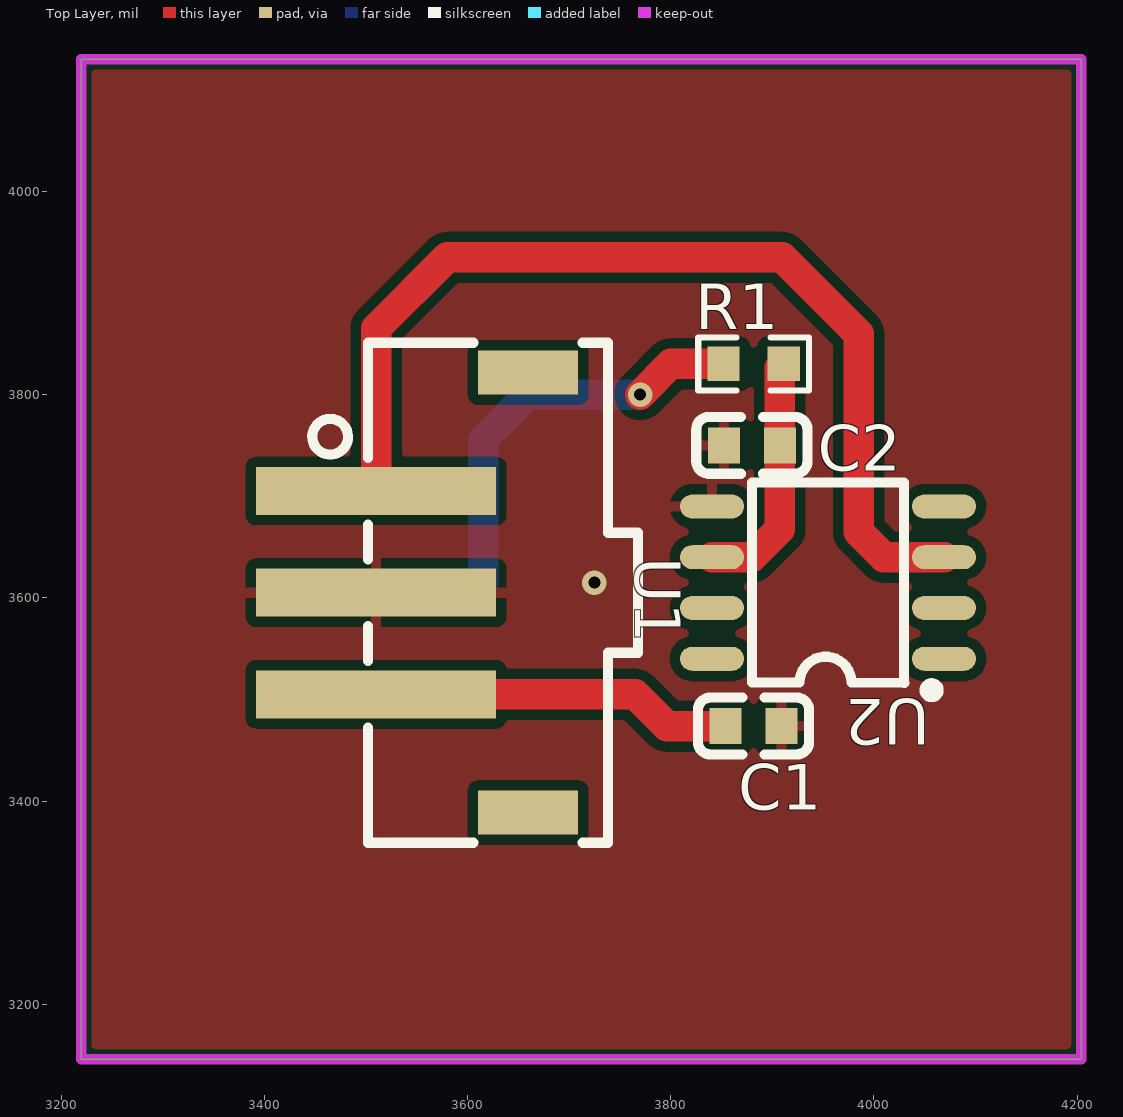
[diagram p0: Top Layer view]
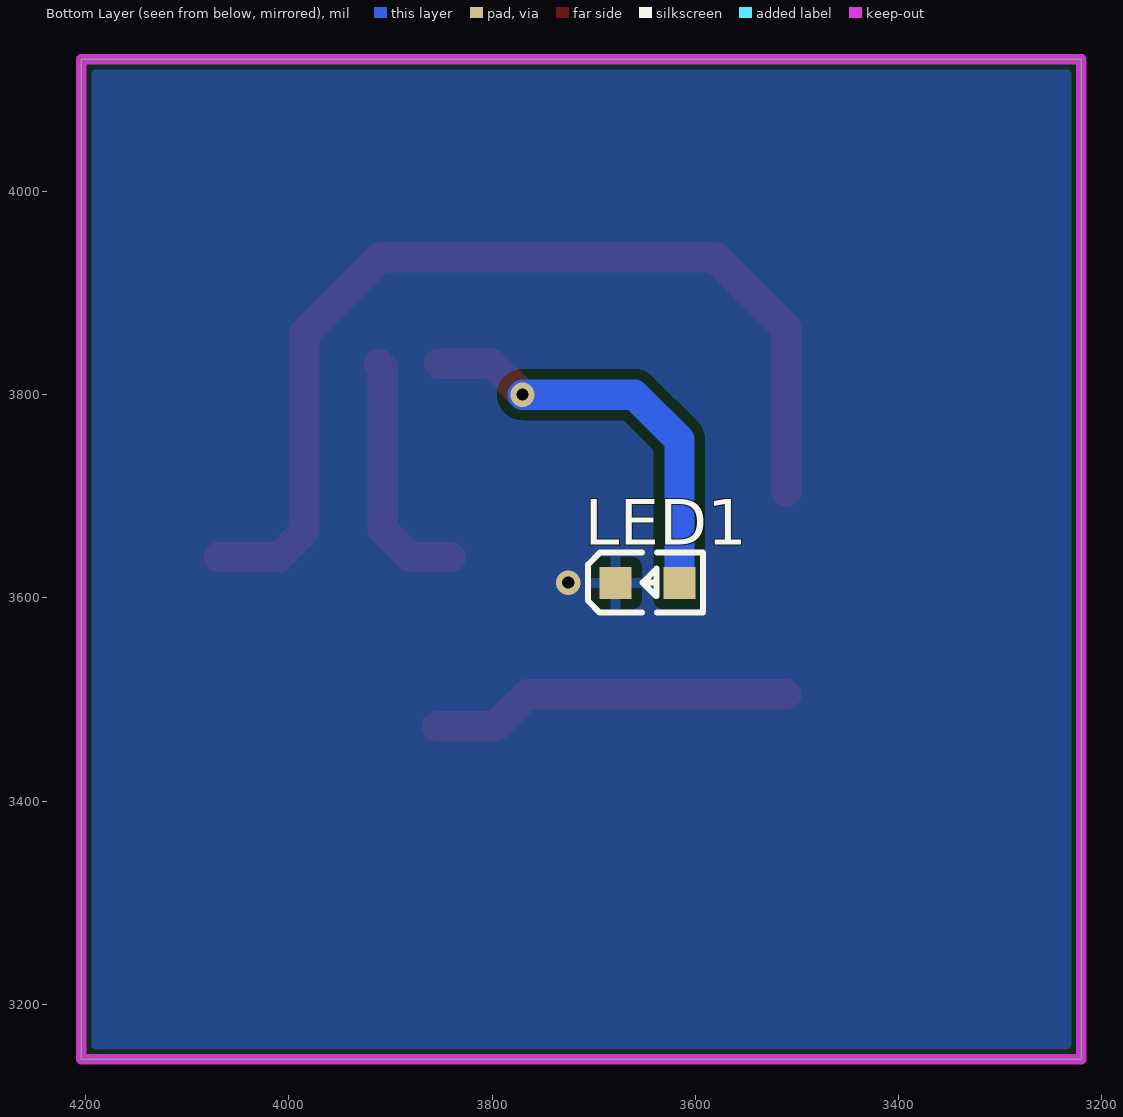
[diagram p1: Bottom Layer view, seen from below]
# Altium PCB MISC51135.pcbdoc
Units mil, origin at the board's own origin, x right, y up, seen from the top; angles counter-clockwise.
Board outline 984.25 x 984.25 mil, 2 copper layers (Top Layer, Bottom Layer), stack 62.206 mil thick; 6 components, 6 nets, 21 pads, 2 vias.

## Layer stack, top to bottom
Top Solder Mask Layer: solder mask 0.394, Dk 3.3
Top Layer: signal copper 1.379
Dielectric1: surface 59.449, FR4, Dk 4.5
Bottom Layer: signal copper 1.378
Bottom Solder Mask Layer: solder mask 0.394, Dk 3.3

## Board outline
3220,4130 3220,3145.75 4204.25,3145.75 4204.25,4130

## Design rules (kind name [scope] priority, off if disabled: settings)
BoardOutlineClearance copperThickness2oz_1 [All] p2 off: genericclearance=7.99 ignorepadtopadclearanceinfootprint=FALSE except(0: Arc-SplitContinuation Track-SplitContinuation SMDPad-SplitContinuation THPad-SplitContinuation Via-SplitContinuation Fill-SplitContinuation Region-SplitContinuation Poly-SplitContinuation Text-SplitContinuation Hole-SplitContinuation; 5.98: Arc-CutoutEdge SMDPad-CutoutEdge THPad-CutoutEdge Via-CutoutEdge Fill-CutoutEdge Region-CutoutEdge Text-CutoutEdge; 6.93: Hole-OutlineEdge Hole-CutoutEdge; 10: Poly-OutlineEdge Poly-CutoutEdge; 11.81: Arc-OutlineEdge Track-OutlineEdge SMDPad-OutlineEdge THPad-OutlineEdge Via-OutlineEdge Fill-OutlineEdge Region-OutlineEdge Text-OutlineEdge Track-CutoutEdge)
BoardOutlineClearance copperThickness1oz_1 [All] p4: genericclearance=4.02 ignorepadtopadclearanceinfootprint=FALSE except(0: Arc-SplitContinuation Track-SplitContinuation SMDPad-SplitContinuation THPad-SplitContinuation Via-SplitContinuation Fill-SplitContinuation Region-SplitContinuation Poly-SplitContinuation Text-SplitContinuation Hole-SplitContinuation; 6: SMDPad-CutoutEdge THPad-CutoutEdge Via-CutoutEdge Fill-CutoutEdge Region-CutoutEdge Text-CutoutEdge; 6.93: Hole-OutlineEdge Hole-CutoutEdge; 10: Poly-OutlineEdge Poly-CutoutEdge; 11.8: Arc-OutlineEdge Track-OutlineEdge SMDPad-OutlineEdge THPad-OutlineEdge Via-OutlineEdge Fill-OutlineEdge Region-OutlineEdge Text-OutlineEdge; 11.81: Arc-CutoutEdge Track-CutoutEdge)
Clearance copperThickness2oz [All] p1 off: gap=7.99 ignorepadtopadclearanceinfootprint=FALSE except(5.98: SMDPad-Track SMDPad-SMDPad THPad-Track SMDPad-THPad THPad-THPad Track-Via SMDPad-Via THPad-Via Via-Via Fill-Track Region-Track Fill-SMDPad Region-SMDPad Fill-THPad Region-THPad Fill-Via Region-Via Fill-Fill Fill-Region Region-Region Arc-Track Arc-SMDPad Arc-THPad Arc-Via Fill-Arc Region-Arc Arc-Arc Text-Track SMDPad-Text Text-THPad Text-Via Fill-Text Region-Text Arc-Text Text-Text; 6.93: Hole-Track Hole-SMDPad Hole-THPad Hole-Via Fill-Hole Region-Hole Hole-Arc Hole-Text; 10: Poly-Track Poly-SMDPad Poly-THPad Poly-Via Poly-Fill Poly-Region Poly-Poly Poly-Arc Poly-Text Poly-Hole)
Clearance copperThickness1oz [All] p3: gap=4.02 ignorepadtopadclearanceinfootprint=FALSE except(5.98: SMDPad-Track SMDPad-SMDPad THPad-Track SMDPad-THPad THPad-THPad Track-Via SMDPad-Via THPad-Via Via-Via Fill-Track Region-Track Fill-SMDPad Region-SMDPad Fill-THPad Region-THPad Fill-Via Region-Via Fill-Fill Fill-Region Region-Region; 6: Arc-Track Arc-SMDPad Arc-THPad Arc-Via Fill-Arc Region-Arc Arc-Arc Text-Track SMDPad-Text Text-THPad Text-Via Fill-Text Region-Text Arc-Text Text-Text; 6.93: Hole-Track Hole-SMDPad Hole-THPad Hole-Via Fill-Hole Region-Hole Hole-Arc Hole-Text; 10: Poly-Track Poly-SMDPad Poly-THPad Poly-Via Poly-Fill Poly-Region Poly-Poly Poly-Arc Poly-Text Poly-Hole)
DiffPairsRouting differentialPair [All] p1: maxlimit=6 minlimit=6 mostfreqgap=6 toplayer_minwidth=5 toplayer_prefwidth=10 toplayer_maxwidth=100 toplayer_mingap=6 toplayer_prefgap=6 toplayer_maxgap=6 bottomlayer_minwidth=5 bottomlayer_prefwidth=10 bottomlayer_maxwidth=100 bottomlayer_mingap=6 bottomlayer_prefgap=6 bottomlayer_maxgap=6 maxuncoupledlength=10
HoleToHoleClearance otherClearance [All] p1: gap=11.81 allowstackedmicrovias=TRUE
Length netLength [All] p1: minlimit=0 maxlimit=0
MatchedLengths netLengthTolerance [All] p1: tolerance=1000
PasteMaskExpansion pasteMaskExpansion [All] p1: expansion=0
PlaneConnect innerPlane [All] p1: planeconnectstyle=Relief reliefexpansion=20 reliefentries=4 reliefconductorwidth=10 reliefairgap=10
PolygonConnect copperRegion [(InNet('GND'))] p1: connectstyle=Relief reliefconductorwidth=10 reliefentries=4 polygonreliefangle="90 Angle" airgapwidth=10 via.connectstyle=Relief via.reliefconductorwidth=10 via.reliefentries=4 via.polygonreliefangle="90 Angle" via.airgapwidth=10
RoutingVias viaSize [All] p1: holewidth=12.01 width=24.02 viastyle="Through Hole" minholewidth=11.81 minwidth=19.68 maxholewidth=248.03 maxwidth=393.7
SolderMaskExpansion solderMaskExpansion [IsVia] p1: expansion=-1000 istentingtop=TRUE
SolderMaskExpansion solderMaskExpansion [All] p2: expansion=2 istentingtop=FALSE
Width copperThickness2oz_2 [All] p1 off: maxlimit=100 minlimit=8 preferedwidth=10
Width copperThickness1oz_2 [All] p2: maxlimit=100 minlimit=5 preferedwidth=10

## Components (designator, comment, footprint, x,y, rotation, side; value= is the part's Value field where it differs from the comment)
C1 "100nF" C0603 3881.65,3473.8 r180 top
C2 "10uF" C0603 3880,3750 r0 top
LED1 "" LED_0603 3645,3615 r180 bottom
R1 "100" R0603 3881.76,3830.23 r0 top
U1 "2.543PIN vertical latching terminal" CONN-SMD_3P-P2.54_C9900012759 3585,3605 r90 top
U2 "ATW62D" SOP-8_L4.9-W3.9-P1.27-LS6.0-TL 3955,3615 r180 top

## Footprints (in the part's own frame and the unit in brackets; to place one, negate y for a bottom-side part, rotate by r counter-clockwise, add the part's x,y. Pads: shape width x height; smd on the part's side, far side on the other; paste and mask are expansions set on the pad)
C0603 [mm]
  rect 0.8x0.9 smd: 1(-0.7,0) 2(0.7,0)
  silkscreen extent -1.39,-0.71 1.39,0.71
CONN-SMD_3P-P2.54_C9900012759 [mm]
  rect 1.2x6 smd paste+0 mask+0.05: 1(2.54,1.9) 2(0,1.9) 3(-2.54,1.9)
  rect 1.1x2.5 smd paste+0 mask+0.05: 4(-5.5,-1.9) 5(5.5,-1.9)
  silkscreen extent -6.25,-4.65 6.25,3.5
LED_0603 [mil]
  rect 31.5x31.5 smd paste+0 mask+2: 1(-33.5,-0.4) 2(29.5,-0.2)
  silkscreen extent -61,-30 53,30
R0603 [mil]
  rect 31.75x34.02 smd paste-3937.01 mask+2: 1(-29.66,0) 2(29.66,0)
  silkscreen extent -55,-26 55,26
SOP-8_L4.9-W3.9-P1.27-LS6.0-TL [mm]
  oval 1.6x0.6 smd: 1(-2.9,1.905) 2(-2.9,0.635) 3(-2.9,-0.635) 4(-2.9,-1.905) 5(2.9,-1.905) 6(2.9,-0.635) 7(2.9,0.635) 8(2.9,1.905)
  silkscreen extent -2.74,-2.5 1.9,2.84

## Via types
v1: diameter 24.02, hole 12, Top Layer to Bottom Layer, 2 vias

## Nets (pads, with @x,y where several pads share a name; then routed paths per layer and width w, separated by ;. In a path a pad name is that pad's centre, name@x,y a point inside that pad or via, vN(x,y) a via of type N, cw(c..) or ccw(c..) an arc to the next point about the centre after c; other vN are vias at no path point)
$1N2: C1.2 U1.3 | length 356.8
  Top Layer w30: U1.3 3765,3505 3796.2,3473.8 C1.2
$1N7: LED1.2 R1.1 | length 408.3
  Top Layer w30: v1(3770,3800) 3800.23,3830.23 R1.1
  Bottom Layer w30: LED1.2 3615.5,3755.5 3660,3800 v1(3770,3800)
GND: C1.1 C2.1 LED1.1 U1.2 U2.5
  other v1: 3725,3615
PWM: U1.1 U2.3 | length 984.5
  Top Layer w30: U1.1 3510.2,3865.2 3580,3935 3910,3935 3985,3860 3985,3665 4010,3640 U2.3
VCC: U2.8
VOUT: C2.2 R1.2 U2.6 | length 242.4
  Top Layer w30: U2.6 3880,3640 3907.56,3667.56 C2.2 3907.56,3826.38 R1.2
pads on no net: U1.4 U1.5 U2.1 U2.2 U2.4 U2.7

## Polygon pours and split planes (outlines as drawn)
GND on Top Layer (solid, remove dead copper, pour order 0): 3025,4230 3025,3025 4270,3025 4270,4230
GND on Bottom Layer (solid, remove dead copper, pour order 2): 3000,4255 3000,3000 4280,3000 4280,4255

## Keep-outs
Board Outline Layer:
  the board outline again, w10